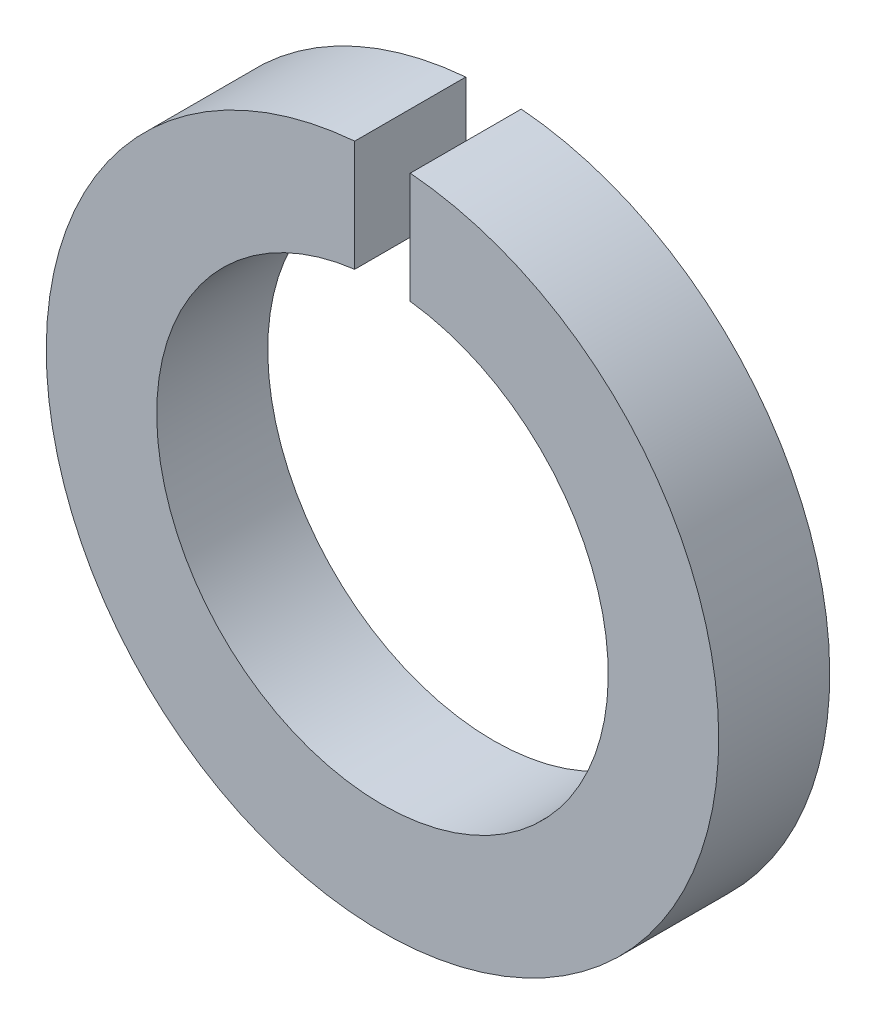
SolidWorks part; units mm, degrees
material "65Mn"
ref_plane "前视基准面" through (0, 0, 0) normal (0, 0, 1) x (1, 0, 0)
ref_plane "上视基准面" through (0, 0, 0) normal (0, 1, 0) x (1, 0, 0)
ref_plane "右视基准面" through (0, 0, 0) normal (1, 0, 0) x (0, 0, -1)
sketch "草图1" plane through (0, 0, 0) normal (0, 0, 1) x (1, 0, 0)
  line L0 (0, 0) -> (0, 103.5317) construction
  line L1 (-1.875, 22.6343) -> (-1.875, 15.1343)
  line L2 (1.875, 22.6343) -> (1.875, 15.1343)
  arc A0 (-1.875, 22.6343) -> (1.875, 22.6343) centre (0, 0) ccw
  arc A2 (-1.875, 15.1343) -> (1.875, 15.1343) centre (0, 0) ccw
extrude "拉伸1" add sketch "草图1" along normal blind 7.5
equation "\"D4@草图1\" = \"m@草图1\" / 2"
